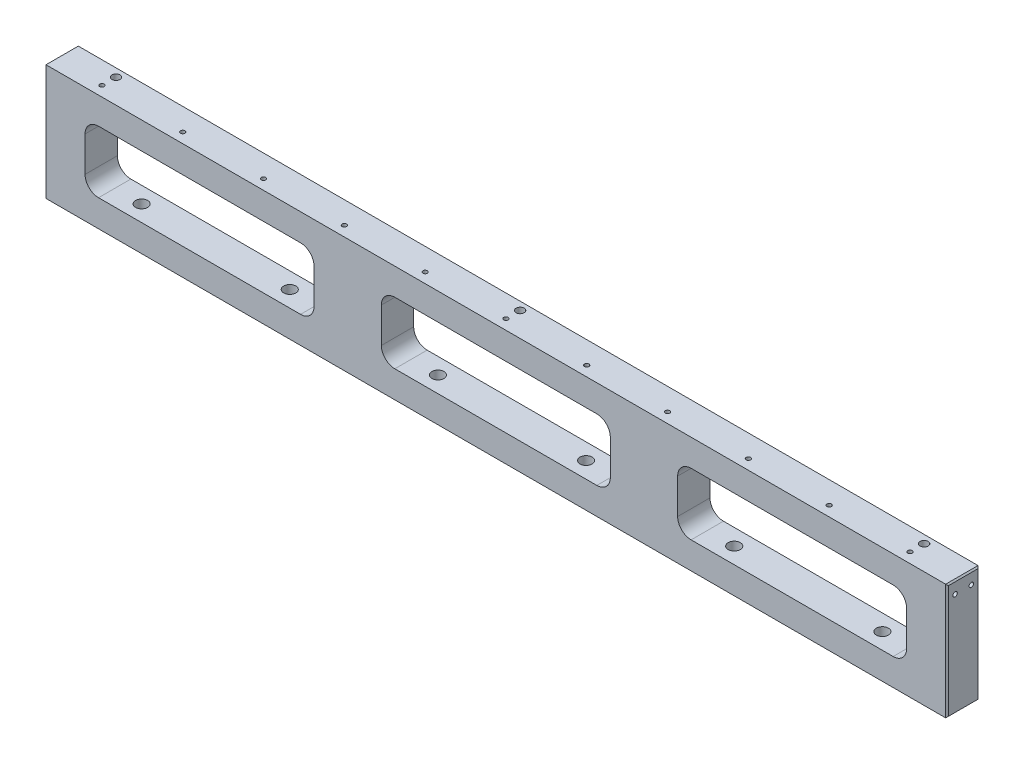
from build123d import *

# Parameters (mm, degrees)
SKETCH1_W                = 670
SKETCH1_H                = 86
BOSS_EXTRUDE1_DEPTH      = 12
CUT_EXTRUDE1_DEPTH       = 339.600059067
M8_CLEARANCE_HOLE1_D     = 9
M8_CLEARANCE_HOLE1_DEPTH = 20
M4_TAPPED_HOLE1_D        = 3.3
M4_TAPPED_HOLE1_DEPTH    = 10.1
M4_TAPPED_HOLE1_TIP      = 0.991420021
DOWEL_HOLE1_D            = 6
DOWEL_HOLE1_DEPTH        = 10.1
DOWEL_HOLE1_TIP          = 1.802581857
CHAMFER1_SIZE            = 1
M4_TAPPED_HOLE2_D        = 3.3
M4_TAPPED_HOLE2_DEPTH    = 10.1
M4_TAPPED_HOLE2_TIP      = 0.991420021
M4_TAPPED_HOLE3_D        = 3.3
M4_TAPPED_HOLE3_DEPTH    = 10.1
M4_TAPPED_HOLE3_TIP      = 0.991420021


with BuildPart() as part:
    # Sketch1 → Boss-Extrude1 (new, symmetric)
    with BuildSketch(Plane.XY):
        Rectangle(SKETCH1_W, SKETCH1_H)
    extrude(amount=BOSS_EXTRUDE1_DEPTH, both=True)

    # Sketch2 → Cut-Extrude1 (cut, through all)
    with BuildSketch(Plane.XY.offset(12)):
        with BuildLine():
            Line((-295, 23), (-145, 23))
            ThreePointArc((-145, 23), (-137.928932188, 20.071067812), (-135, 13))
            Line((-135, 13), (-135, -13))
            ThreePointArc((-135, -13), (-137.928932188, -20.071067812), (-145, -23))
            Line((-145, -23), (-295, -23))
            ThreePointArc((-295, -23), (-302.071067812, -20.071067812), (-305, -13))
            Line((-305, -13), (-305, 13))
            ThreePointArc((-305, 13), (-302.071067812, 20.071067812), (-295, 23))
        make_face()
        with BuildLine():
            Line((-75, 23), (75, 23))
            ThreePointArc((75, 23), (82.071067812, 20.071067812), (85, 13))
            Line((85, 13), (85, -13))
            ThreePointArc((85, -13), (82.071067812, -20.071067812), (75, -23))
            Line((75, -23), (-75, -23))
            ThreePointArc((-75, -23), (-82.071067812, -20.071067812), (-85, -13))
            Line((-85, -13), (-85, 13))
            ThreePointArc((-85, 13), (-82.071067812, 20.071067812), (-75, 23))
        make_face()
        with BuildLine():
            Line((145, 23), (295, 23))
            ThreePointArc((295, 23), (302.071067812, 20.071067812), (305, 13))
            Line((305, 13), (305, -13))
            ThreePointArc((305, -13), (302.071067812, -20.071067812), (295, -23))
            Line((295, -23), (145, -23))
            ThreePointArc((145, -23), (137.928932188, -20.071067812), (135, -13))
            Line((135, -13), (135, 13))
            ThreePointArc((135, 13), (137.928932188, 20.071067812), (145, 23))
        make_face()
    extrude(amount=-CUT_EXTRUDE1_DEPTH, mode=Mode.SUBTRACT)

    # M8 Clearance Hole1
    with Locations(Plane(origin=(0, -43, 0), x_dir=(-1, 0, 0), z_dir=(0, -1, 0))):
        with Locations((-275, 0), (275, 0), (165, 0), (55, 0), (-55, 0), (-165, 0)):
            Hole(M8_CLEARANCE_HOLE1_D / 2, depth=M8_CLEARANCE_HOLE1_DEPTH)

    # M4 Tapped Hole1
    with Locations(Plane(origin=(0, 43, 0), x_dir=(1, 0, 0), z_dir=(0, 1, 0))):
        with Locations((-300, -4.5), (-240, -4.5), (-180, -4.5), (-120, -4.5), (-60, -4.5), (0, -4.5), (60, -4.5), (120, -4.5), (180, -4.5), (240, -4.5), (300, -4.5)):
            Hole(M4_TAPPED_HOLE1_D / 2, depth=M4_TAPPED_HOLE1_DEPTH)
            with Locations((0, 0, -(M4_TAPPED_HOLE1_DEPTH + M4_TAPPED_HOLE1_TIP / 2))):  # 118° drill point
                Cone(0, M4_TAPPED_HOLE1_D / 2, M4_TAPPED_HOLE1_TIP, mode=Mode.SUBTRACT)

    # Dowel Hole1
    with Locations(Plane(origin=(0, 43, 0), x_dir=(1, 0, 0), z_dir=(0, 1, 0))):
        with Locations((300, 6), (-300, 6), (0, 6)):
            Hole(DOWEL_HOLE1_D / 2, depth=DOWEL_HOLE1_DEPTH)
            with Locations((0, 0, -(DOWEL_HOLE1_DEPTH + DOWEL_HOLE1_TIP / 2))):  # 118° drill point
                Cone(0, DOWEL_HOLE1_D / 2, DOWEL_HOLE1_TIP, mode=Mode.SUBTRACT)

    # Chamfer1
    chamfer1_edges = [part.edges().sort_by_distance(p)[0] for p in [
        (-335, 0, 12),
        (335, 0, 12),
        (-335, 0, -12),
        (335, 0, -12),
        (335, -43, 0),
        (-335, -43, 0),
        (-335, 43, 0),
        (335, 43, 0),
    ]]
    chamfer(chamfer1_edges, length=CHAMFER1_SIZE)

    # M4 Tapped Hole2
    with Locations(Plane.ZY.offset(335)):
        with Locations((6, 34), (-6, 34)):
            Hole(M4_TAPPED_HOLE2_D / 2, depth=M4_TAPPED_HOLE2_DEPTH)
            with Locations((0, 0, -(M4_TAPPED_HOLE2_DEPTH + M4_TAPPED_HOLE2_TIP / 2))):  # 118° drill point
                Cone(0, M4_TAPPED_HOLE2_D / 2, M4_TAPPED_HOLE2_TIP, mode=Mode.SUBTRACT)

    # M4 Tapped Hole3
    with Locations(Plane(origin=(335, 0, 0), x_dir=(0, 0, -1), z_dir=(1, 0, 0))):
        with Locations((-6, 34), (6, 34)):
            Hole(M4_TAPPED_HOLE3_D / 2, depth=M4_TAPPED_HOLE3_DEPTH)
            with Locations((0, 0, -(M4_TAPPED_HOLE3_DEPTH + M4_TAPPED_HOLE3_TIP / 2))):  # 118° drill point
                Cone(0, M4_TAPPED_HOLE3_D / 2, M4_TAPPED_HOLE3_TIP, mode=Mode.SUBTRACT)


solid = part.part
